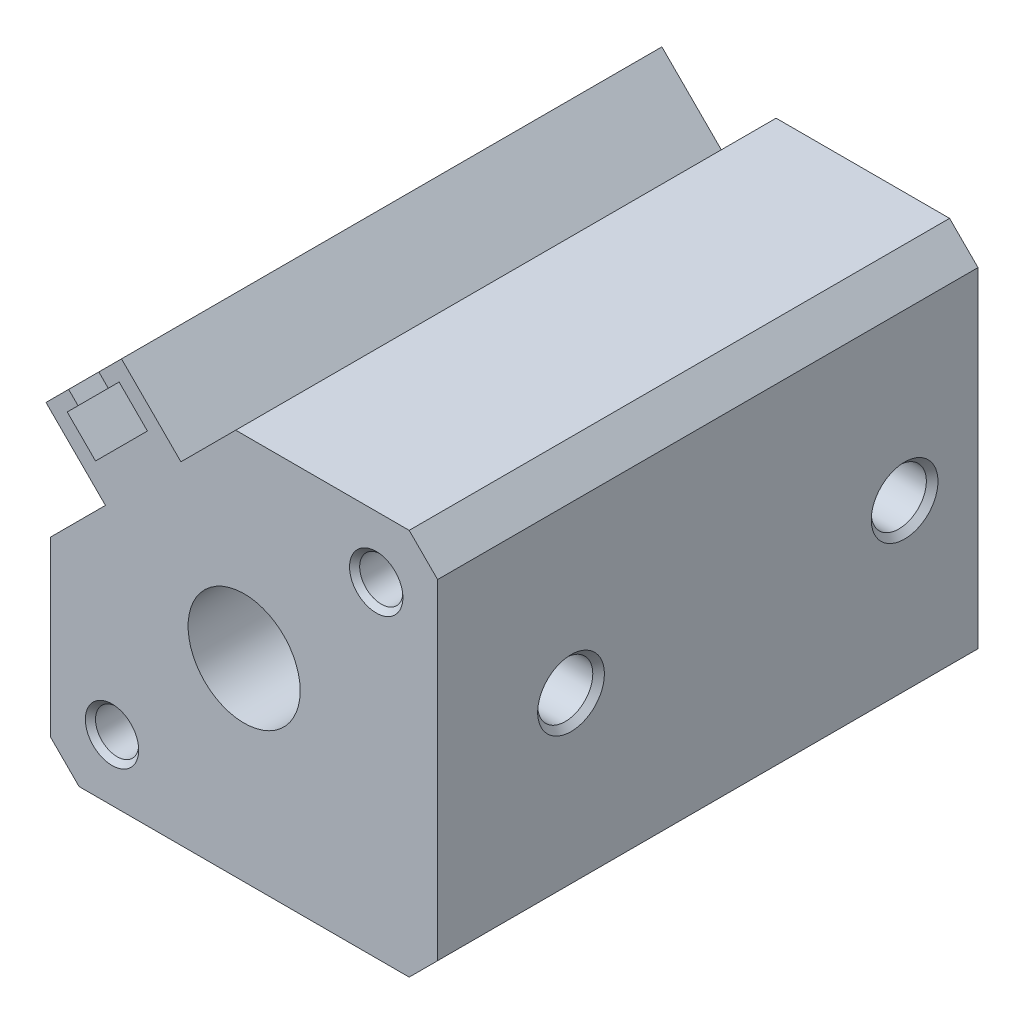
from build123d import *

# Parameters (mm, degrees)
EXTRUDE_1_DEPTH     = 40.5
SKETCH_6_R          = 4.2
CUT_EXTRUDE_1_DEPTH = 20


with BuildPart() as part:
    # 草图1 → 凸台-拉伸1 (new body)
    with BuildSketch(Plane.XY):
        Polygon((-14.849242405, 9.192388155), (-10.394469683, 4.737615434), (-14.5, 0.632085117), (-14.5, -12.370057685), (-12.370057685, -14.5), (12.370057685, -14.5), (14.5, -12.370057685), (14.5, 12.370057685), (12.370057685, 14.5), (-0.632085117, 14.5), (-4.737615434, 10.394469683), (-9.192388155, 14.849242405), (-10.88944443, 13.15218613), (-10.182337649, 12.445079349), (-9.369164851, 13.258252147), (-7.247844507, 11.136931804), (-11.136931804, 7.247844507), (-13.258252147, 9.369164851), (-12.445079349, 10.182337649), (-13.15218613, 10.88944443), align=None)
    extrude(amount=-EXTRUDE_1_DEPTH)

    # 草图2 → 切除-旋转1 (revolve, cut)
    with BuildSketch(Plane(origin=(0, 0, 0), x_dir=(1, 0, 0), z_dir=(0, 1, 0)), mode=Mode.PRIVATE) as cut_revolve_1_sk:
        Polygon((8.5, 10), (8.5, 12.065), (14.065, 12.065), (15, 13), (15, 10), align=None)
    revolve(cut_revolve_1_sk.sketch.rotate(Axis((15, 0, -10), (-1, 0, 0)), 180), axis=Axis((15, 0, -10), (-1, 0, 0)), mode=Mode.SUBTRACT)

    # 草图3 → 切除-旋转2 (revolve, cut)
    with BuildSketch(Plane(origin=(0, 0, 0), x_dir=(1, 0, 0), z_dir=(0, 1, 0)), mode=Mode.PRIVATE) as cut_revolve_2_sk:
        Polygon((8.5, 35), (8.5, 37.065), (14.065, 37.065), (15, 38), (15, 35), align=None)
    revolve(cut_revolve_2_sk.sketch.rotate(Axis((15, 0, -35), (-1, 0, 0)), 180), axis=Axis((15, 0, -35), (-1, 0, 0)), mode=Mode.SUBTRACT)

    # 草图4 → 切除-旋转3 (revolve, cut)
    with BuildSketch(Plane(origin=(0, 0, 0), x_dir=(-0.7071067811865475, -0.7071067811865477, 0), z_dir=(0.7071067811865477, -0.7071067811865475, 0)), mode=Mode.PRIVATE) as cut_revolve_3_sk:
        Polygon((-14, -0.5), (-16.5, -0.5), (-15.62, 0.38), (-15.62, 40.12), (-16.5, 41), (-14, 41), align=None)
    revolve(cut_revolve_3_sk.sketch.rotate(Axis((9.899494937, 9.899494937, -41), (0, 0, 1)), 315), axis=Axis((9.899494937, 9.899494937, -41), (0, 0, 1)), mode=Mode.SUBTRACT)

    # 草图5 → 切除-旋转4 (revolve, cut)
    with BuildSketch(Plane(origin=(0, 0, 0), x_dir=(-0.7071067811865475, -0.7071067811865477, 0), z_dir=(0.7071067811865477, -0.7071067811865475, 0)), mode=Mode.PRIVATE) as cut_revolve_4_sk:
        Polygon((14, -0.5), (11.5, -0.5), (12.38, 0.38), (12.38, 40.12), (11.5, 41), (14, 41), align=None)
    revolve(cut_revolve_4_sk.sketch.rotate(Axis((-9.899494937, -9.899494937, -41), (0, 0, 1)), 315), axis=Axis((-9.899494937, -9.899494937, -41), (0, 0, 1)), mode=Mode.SUBTRACT)

    # 草图6 → 切除-拉伸1 (cut)
    with BuildSketch(Plane.XY):
        Circle(SKETCH_6_R)
    extrude(amount=-CUT_EXTRUDE_1_DEPTH, mode=Mode.SUBTRACT)


solid = part.part
